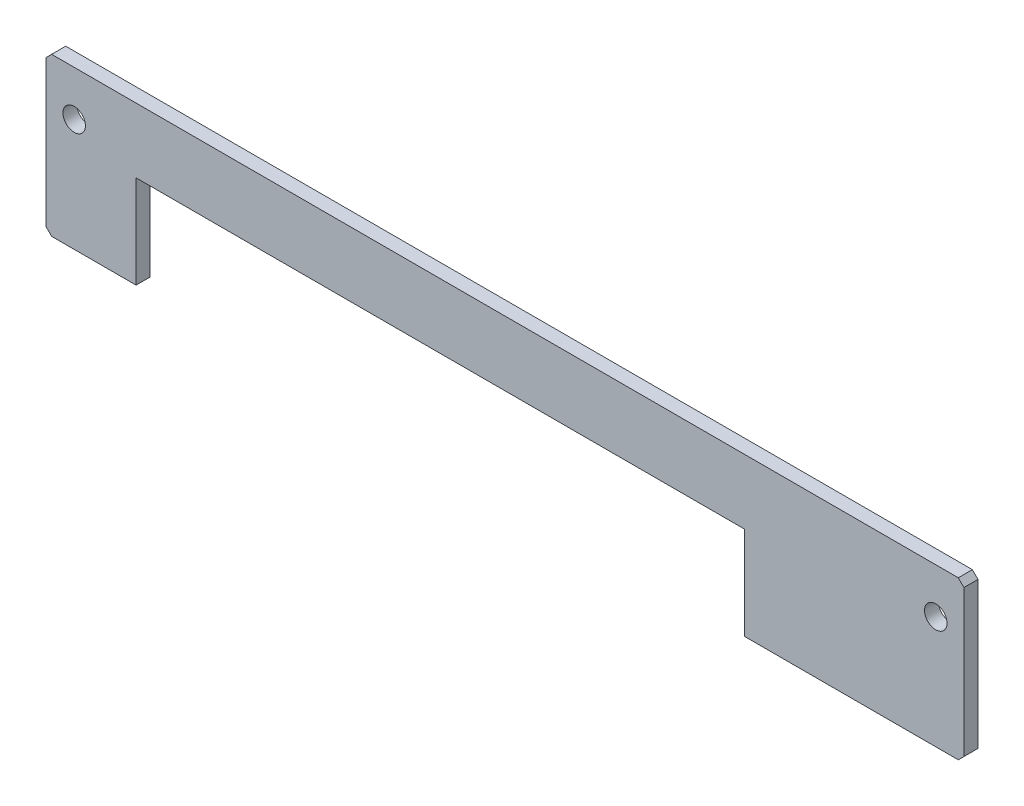
from build123d import *

# Parameters (mm, degrees)
EXTRUDE_1_DEPTH          = 25
CHAMFER_1_SIZE           = 10
CUT_EXTRUDE_1_DEPTH      = 1655.063178963
CUT_EXTRUDE_1_DEPTH_BACK = 1655.063178963
SKETCH_2_R               = 20


with BuildPart() as part:
    # 草图1 → 凸台-拉伸1 (new body)
    with BuildSketch(Plane.XY):
        Polygon((160, -280), (0, -280), (0, 0), (1630, 0), (1630, -280), (1240, -280), (1240, -115), (160, -115), align=None)
    extrude(amount=EXTRUDE_1_DEPTH)

    # 倒角1
    chamfer_1_edges = [part.edges().sort_by_distance(p)[0] for p in [
        (0, -280, 12.5),
        (0, 0, 12.5),
        (1630, 0, 12.5),
        (1630, -280, 12.5),
    ]]
    chamfer(chamfer_1_edges, length=CHAMFER_1_SIZE)

    # 草图2 → 切除-拉伸1 (cut, two sides: drawn at the far end of the back side and taken through both)
    with BuildSketch(Plane.XY.offset(25).offset(-CUT_EXTRUDE_1_DEPTH_BACK)):
        with Locations((50, -80)):
            Circle(SKETCH_2_R)
        with Locations((1580, -80)):
            Circle(SKETCH_2_R)
    extrude(amount=CUT_EXTRUDE_1_DEPTH + CUT_EXTRUDE_1_DEPTH_BACK, mode=Mode.SUBTRACT)


solid = part.part
